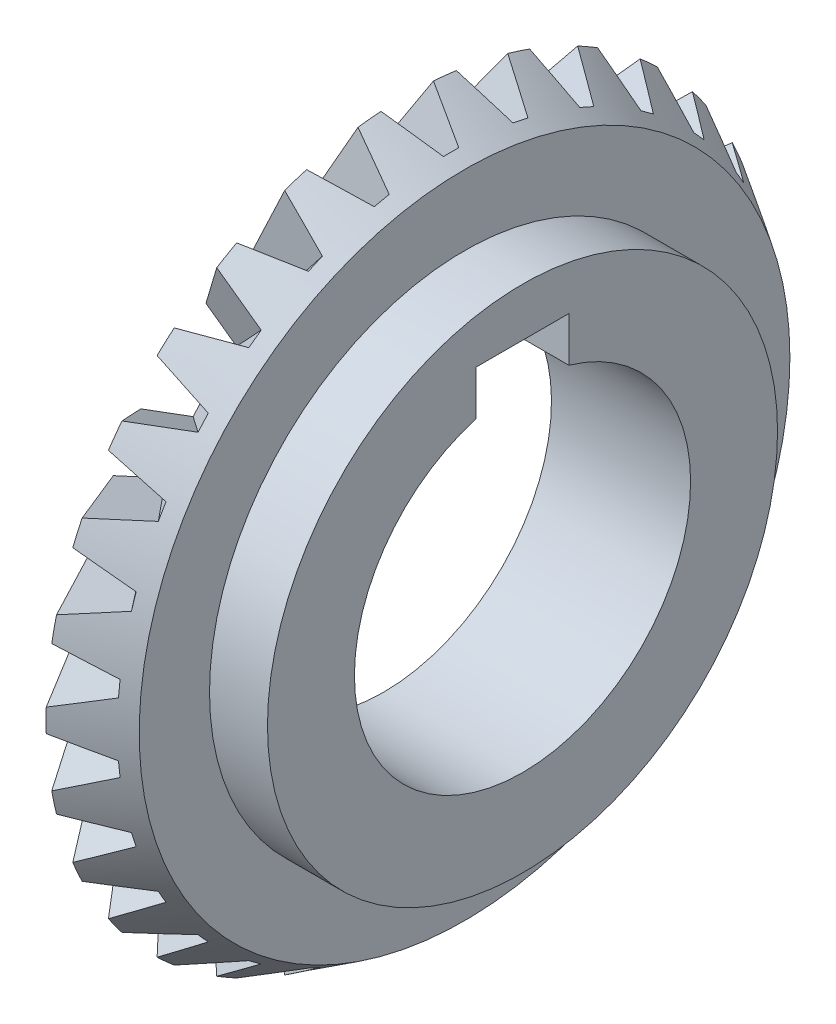
from build123d import *

# Parameters (mm, degrees)
CIRPATTERN1_COUNT  = 30
SKETCH5_W          = 8
SKETCH5_H          = 6.6
CUT_EXTRUDE1_DEPTH = 30


with BuildPart() as part:
    # Sketch1 → Revolve1 (revolve)
    with BuildSketch(Plane.XY, mode=Mode.PRIVATE) as revolve1_sk:
        Polygon((0, 14.5), (0, 22), (-5, 22), (-5, 28.066423399), (-9.948196016, 31.15), (-16, 21.438708135), (-12, 18.946020625), (-12, 14.5), align=None)
    revolve(revolve1_sk.sketch.rotate(Axis((0, 0, 0), (-1, 0, 0)), 90), axis=Axis((0, 0, 0), (-1, 0, 0)))

    # Sketch3 → Cut-Loft1 section 0
    with BuildSketch(Plane(origin=(-8.277529798, 30.108887796, 0), x_dir=(0.8486948816015439, -0.5288827828010112, 0), z_dir=(0.5288827828010112, 0.8486948816015439, 0)), mode=Mode.PRIVATE) as cut_loft1_s0:
        with BuildLine():
            Line((-6.839880107, 4.059512765), (-6.839880107, -4.059512765))
            Line((-6.839880107, -4.059512765), (2.5, -0.660074414))
            Line((2.5, -0.660074414), (2.5, 0.660074414))
            Line((2.5, 0.660074414), (-6.839880107, 4.059512765))
        make_face()
    cut_loft1 = loft([Vertex(-29.36, 0, 0), cut_loft1_s0.sketch], mode=Mode.SUBTRACT)

    # CirPattern1: Cut-Loft1 ×30 about axis
    cirpattern1_axis = Axis((0, 0, 0), (1, 0, 0))
    for i in range(1, CIRPATTERN1_COUNT):
        add(cut_loft1.rotate(cirpattern1_axis, i * 360 / CIRPATTERN1_COUNT), mode=Mode.SUBTRACT)

    # Sketch5 → Cut-Extrude1 (cut)
    with BuildSketch(Plane.ZY.offset(12)):
        with Locations((0, 14.5)):
            Rectangle(SKETCH5_W, SKETCH5_H)
    extrude(amount=-CUT_EXTRUDE1_DEPTH, mode=Mode.SUBTRACT)


solid = part.part
